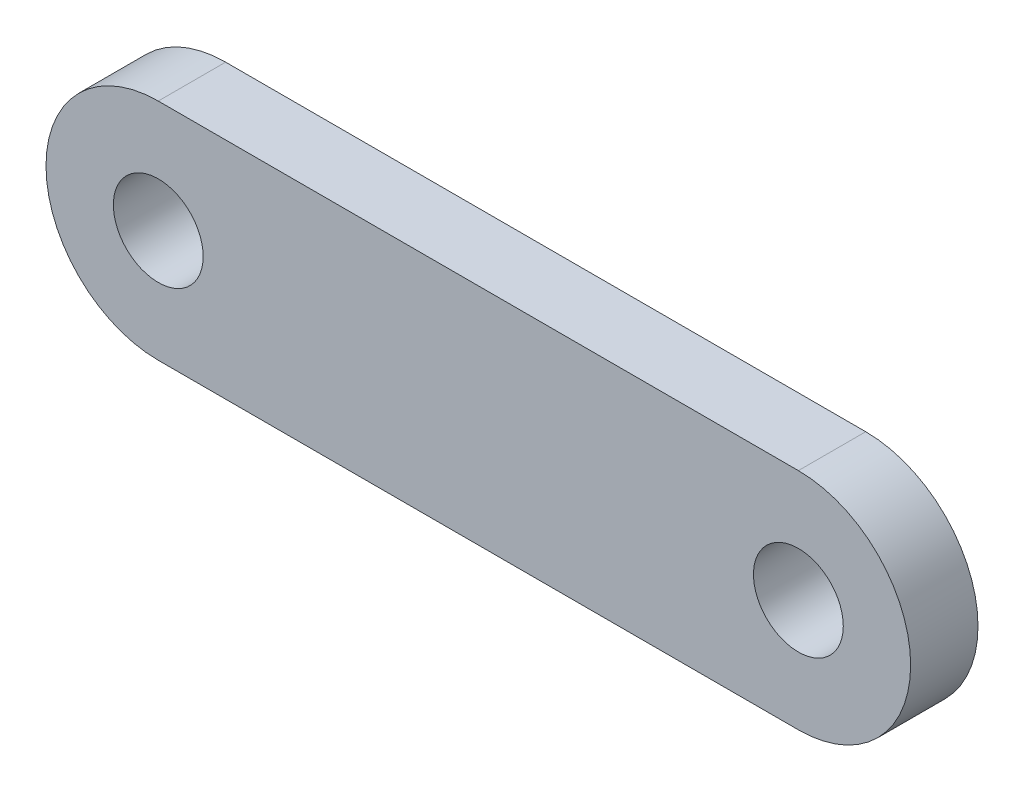
SolidWorks part; units mm, degrees
ref_plane "Front Plane" through (0, 0, 0) normal (0, 0, 1) x (1, 0, 0)
ref_plane "Top Plane" through (0, 0, 0) normal (0, 1, 0) x (1, 0, 0)
ref_plane "Right Plane" through (0, 0, 0) normal (1, 0, 0) x (0, 0, -1)
sketch "Sketch1" plane through (0, 0, 0) normal (0, 0, 1) x (1, 0, 0)
  line L0 (3.3, 0) -> (-3.3, 0) construction
  line L1 (0, 10) -> (57.02, 10)
  line L2 (0, 0) -> (158.2009, 0) construction
  line L3 (0, -10) -> (57.02, -10)
  arc A0 (0, 10) -> (0, -10) centre (0, 0) ccw
  arc A1 (57.02, -10) -> (57.02, 10) centre (57.02, 0) ccw
  dimension "D1" = 57.02
  dimension "D2" = 20
  dimension "D3" = 20
extrude "Boss-Extrude1" add sketch "Sketch1" along normal blind 6
sketch "Sketch2" plane through (0, 0, 6) normal (0, 0, 1) x (1, 0, 0)
  circle A0 centre (0, 0) radius 4
  circle A1 centre (57.02, 0) radius 4
  dimension "D1" = 8
  dimension "D2" = 8
extrude "Cut-Extrude1" cut sketch "Sketch2" against normal blind 95
